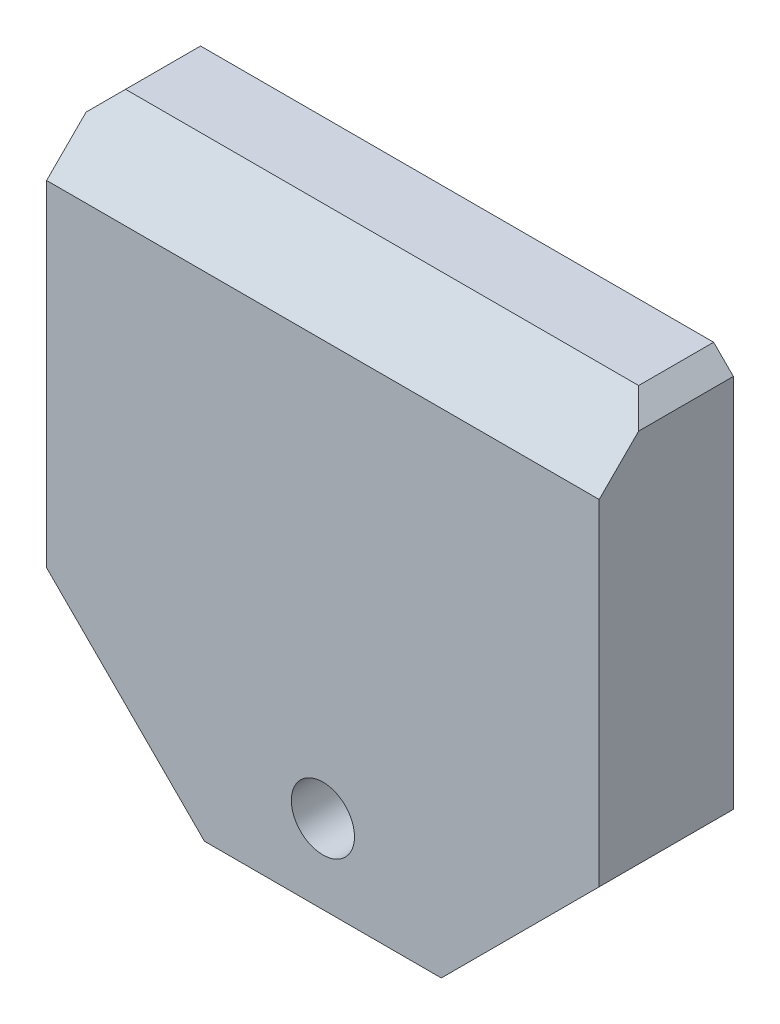
SolidWorks part; units mm, degrees
material "Q235A"
ref_plane "Front Plane" through (0, 0, 0) normal (0, 0, 1) x (1, 0, 0)
ref_plane "Top Plane" through (0, 0, 0) normal (0, 1, 0) x (1, 0, 0)
ref_plane "Right Plane" through (0, 0, 0) normal (1, 0, 0) x (0, 0, -1)
sketch "Sketch1" plane through (0, 0, 0) normal (0, 0, 1) x (1, 0, 0)
  line L1 (70, -70) -> (-70, -70)
  line L2 (70, -70) -> (70, 70)
  line L3 (70, 70) -> (-70, 70)
  line L4 (-70, -70) -> (-70, 70)
  line L5 (70, -70) -> (-70, 70) construction
  line L6 (70, 70) -> (-70, -70) construction
  point P0 (0, 0)
  dimension "D1" = 140
  dimension "D2" = 140
extrude "Boss-Extrude1" add sketch "Sketch1" along normal blind 34
sketch "Sketch3" plane through (0, 0, 34) normal (0, 0, 1) x (1, 0, 0)
  line L0 (0, 70) -> (0, -94.2409) construction
  line L1 (70, 70) -> (-70, 70) construction
  circle A2 centre (0, -50) radius 8
  dimension "D4" = 16
  dimension "D5" = 120
extrude "Cut-Extrude3" cut sketch "Sketch3" against normal through all contours A2
chamfer "Chamfer1" distance 5 angle 45 2 edges at (70, 70, 17) (-70, 70, 17)
chamfer "Chamfer2" distance 15 angle 45 1 edges at (0, 70, 34)
chamfer "Chamfer3" distance 40 angle 45 2 edges at (70, -70, 17) (-70, -70, 17)
